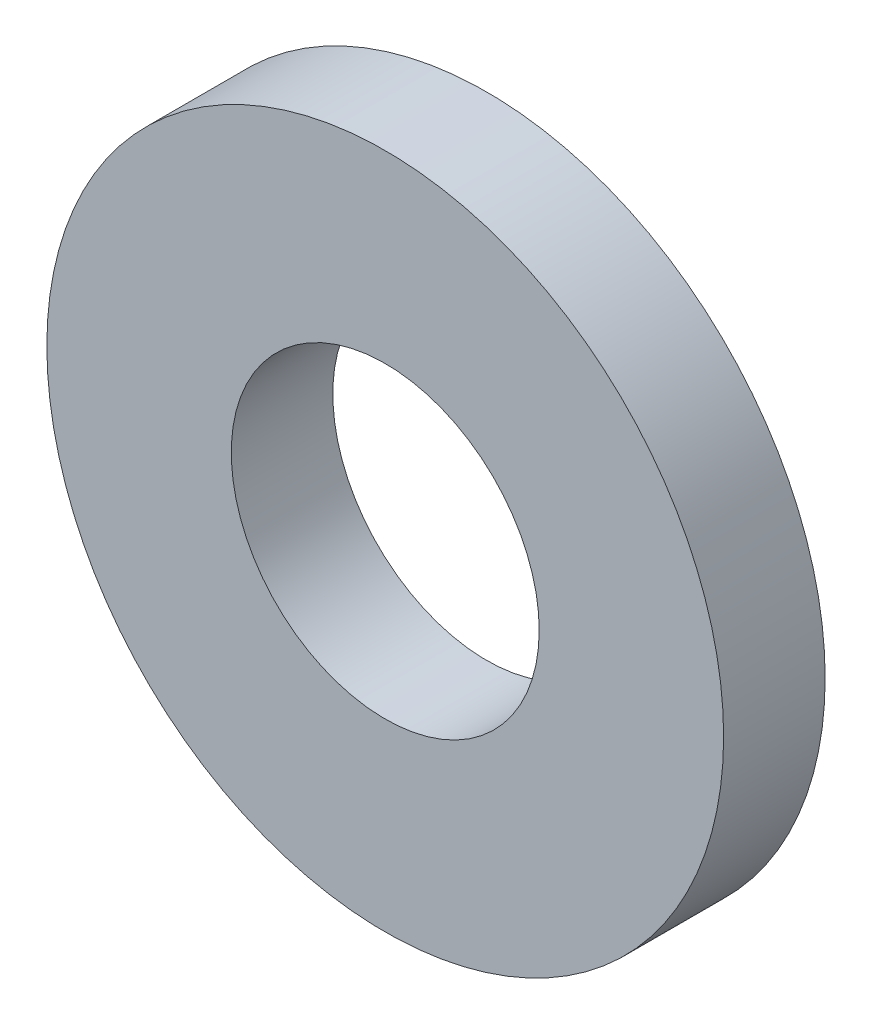
from build123d import *

# Parameters (mm, degrees)
SKETCH_1_R      = 50
SKETCH_1_R_2    = 22.75
EXTRUDE_1_DEPTH = 15


with BuildPart() as part:
    # 草图1 → 凸台-拉伸1 (new body)
    with BuildSketch(Plane.XY):
        Circle(SKETCH_1_R)
        Circle(SKETCH_1_R_2, mode=Mode.SUBTRACT)
    extrude(amount=EXTRUDE_1_DEPTH)


solid = part.part
